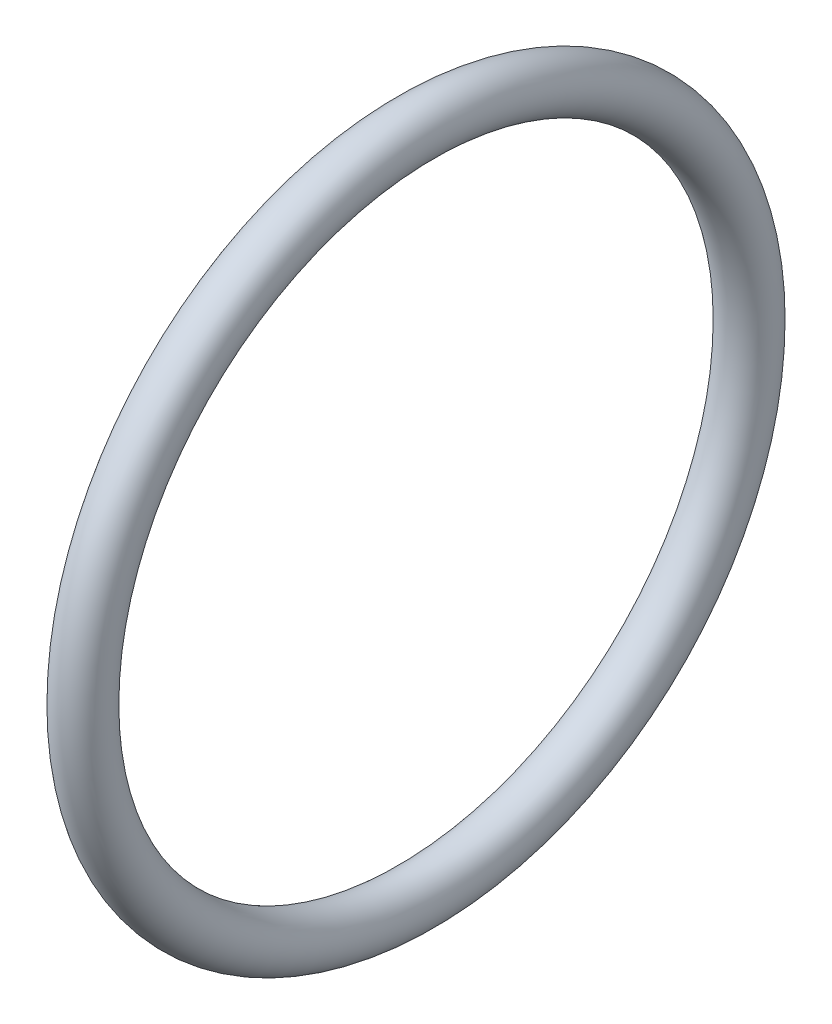
from build123d import *

# Parameters (mm, degrees)
SKETCH1_R = 1.325


with BuildPart() as part:
    # Sketch1 → Revolve1 (revolve)
    with BuildSketch(Plane.XY, mode=Mode.PRIVATE) as revolve1_sk:
        with Locations((5, 17.35)):
            Circle(SKETCH1_R)
    revolve(revolve1_sk.sketch.rotate(Axis((0, 0, 0), (1, 0, 0)), 90), axis=Axis((0, 0, 0), (1, 0, 0)))


solid = part.part
